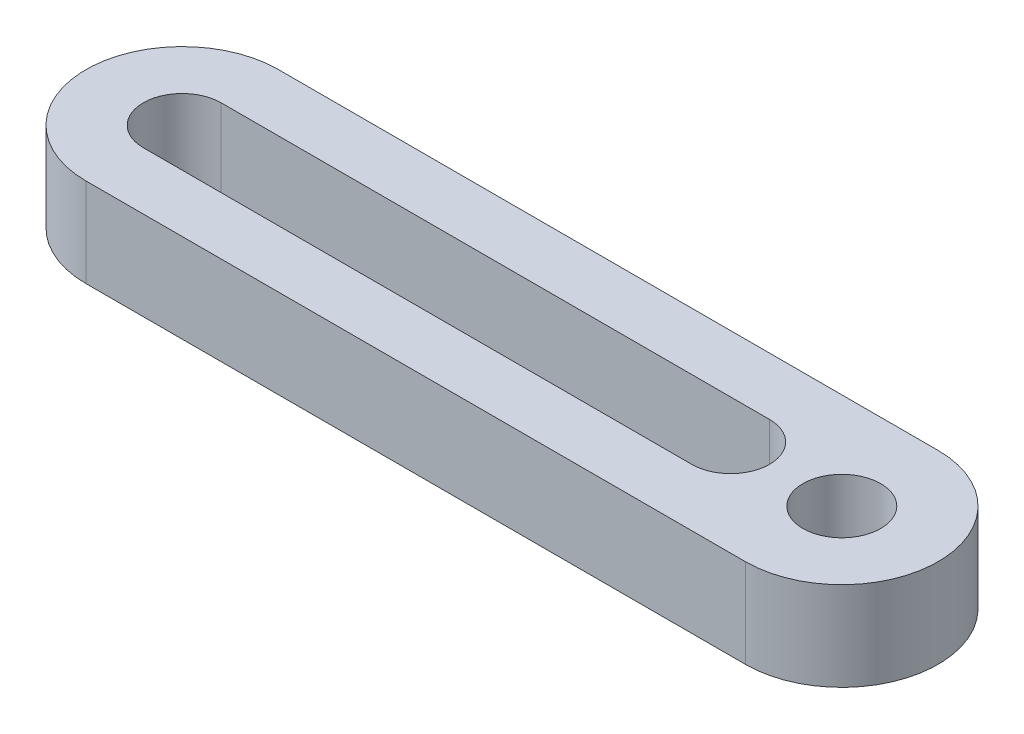
SolidWorks part; units mm, degrees
material "Q235A"
ref_plane "Front Plane" through (0, 0, 0) normal (0, 0, 1) x (1, 0, 0)
ref_plane "Top Plane" through (0, 0, 0) normal (0, 1, 0) x (1, 0, 0)
ref_plane "Right Plane" through (0, 0, 0) normal (1, 0, 0) x (0, 0, -1)
sketch "Sketch1" plane through (0, 0, 0) normal (0, 1, 0) x (1, 0, 0)
  line L0 (-44.5, 0) -> (44.5, 0) construction
  line L1 (-44.5, 13) -> (44.5, 13)
  line L2 (-44.5, -13) -> (44.5, -13)
  line L3 (-44.5, 0) -> (29.5, 0) construction
  line L4 (-44.5, 5.25) -> (29.5, 5.25)
  line L5 (-44.5, -5.25) -> (29.5, -5.25)
  arc A0 (-44.5, 13) -> (-44.5, -13) centre (-44.5, 0) ccw
  arc A1 (44.5, -13) -> (44.5, 13) centre (44.5, 0) ccw
  arc A2 (-44.5, 5.25) -> (-44.5, -5.25) centre (-44.5, 0) ccw
  arc A3 (29.5, -5.25) -> (29.5, 5.25) centre (29.5, 0) ccw
  circle A4 centre (44.5, 0) radius 5.25
  point P2 (0, 0)
  point P10 (-7.5, 0)
  dimension "D5" = 10.5
  dimension "D1" = 26
  dimension "D2" = 115
  dimension "D3" = 10.5
  dimension "D4" = 74
extrude "Boss-Extrude1" add sketch "Sketch1" along normal mid plane 12
